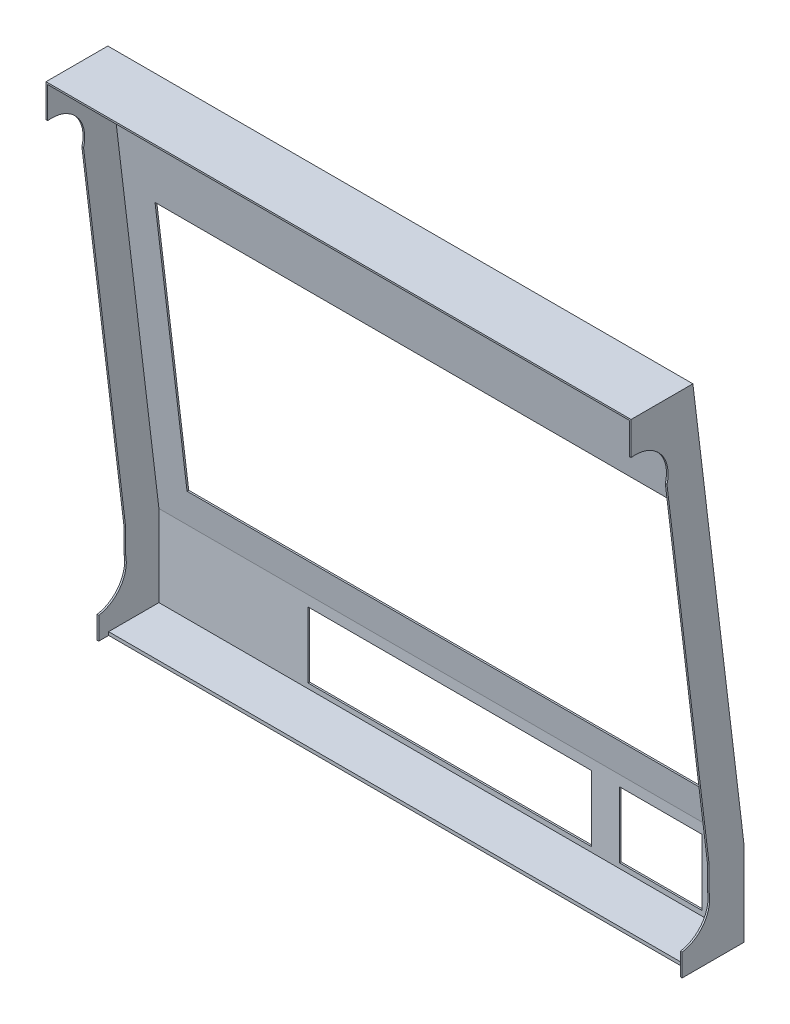
from build123d import *

# Parameters (mm, degrees)
BOSS_EXTRUDE1_DEPTH = 2
BOSS_EXTRUDE2_DEPTH = 706
SKETCH3_W           = 706
SKETCH3_H           = 73
CUT_EXTRUDE1_DEPTH  = 940.955850027
BOSS_EXTRUDE3_START = 2
BOSS_EXTRUDE3_DEPTH = 2
CUT_EXTRUDE2_REACH  = 951.714
SKETCH5_W           = 628
SKETCH5_H           = 323
SKETCH6_W           = 100
SKETCH6_H           = 80
SKETCH6_W_2         = 344
CUT_EXTRUDE3_DEPTH  = 2
SKETCH7_W           = 706
SKETCH7_H           = 4
BOSS_EXTRUDE4_DEPTH = 61


with BuildPart() as part:
    # Sketch1 → Boss-Extrude1 (new body)
    with BuildSketch(Plane(origin=(0, 0, 0), x_dir=(0, 0, -1), z_dir=(1, 0, 0))):
        with BuildLine():
            Line((0, 0), (-75, 0))
            Line((-75, 0), (-75, -40))
            ThreePointArc((-75, -40), (-39.844354311, -53.471133381), (-31.447716035, -90.171096924))
            Line((-31.447716035, -90.171096924), (19.696734432, -515))
            Line((19.696734432, -515), (19.696734432, -543.691772505))
            ThreePointArc((19.696734432, -543.691772505), (13.304376378, -574.16353688), (-13, -590.820981133))
            Line((-13, -590.820981133), (-13, -618))
            Line((-13, -618), (62, -618))
            Line((62, -618), (62, -515))
            Line((62, -515), (0, 0))
        make_face()
    extrude(amount=BOSS_EXTRUDE1_DEPTH)

    # Sketch2 → Boss-Extrude2 (add)
    with BuildSketch(Plane.ZY):
        Polygon((13, -618), (-62, -618), (-62, -515), (0, 0), (75, 0), (75, -2), (1.773664518, -2), (-60, -515.119955274), (-60, -616), (13, -616), align=None)
    extrude(amount=BOSS_EXTRUDE2_DEPTH)

    # Sketch3 → Cut-Extrude1 (cut, through all)
    with BuildSketch(Plane(origin=(0, -616, 0), x_dir=(1, 0, 0), z_dir=(0, 1, 0))):
        with Locations((-353, 23.5)):
            Rectangle(SKETCH3_W, SKETCH3_H)
    extrude(amount=-CUT_EXTRUDE1_DEPTH, mode=Mode.SUBTRACT)

    # Sketch4 → Boss-Extrude3 (add)
    with BuildSketch(Plane.ZY.offset(706).offset(BOSS_EXTRUDE3_START)):
        with BuildLine():
            Line((-19.696734432, -543.691772505), (-19.696734432, -515))
            Line((-19.696734432, -515), (31.447716035, -90.171096924))
            ThreePointArc((31.447716035, -90.171096924), (39.844354311, -53.471133381), (75, -40))
            Line((75, -40), (75, 0))
            Line((75, 0), (0, 0))
            Line((0, 0), (-62, -515))
            Line((-62, -515), (-62, -618))
            Line((-62, -618), (13, -618))
            Line((13, -618), (13, -590.820981133))
            ThreePointArc((13, -590.820981133), (-13.304376378, -574.16353688), (-19.696734432, -543.691772505))
        make_face()
    extrude(amount=-BOSS_EXTRUDE3_DEPTH)

    # Cut-Extrude2: up to this plane
    cut_extrude2_end = Plane(origin=(-706, -515.119955274, -60), z_dir=(0, 0.1195253040577556, -0.9928311546732914))
    # Sketch5 → Cut-Extrude2 (cut, up to the surface)
    with BuildSketch(Plane(origin=(0, 0, -62), x_dir=(-1, 0, 0), z_dir=(0, 0, -1)), mode=Mode.PRIVATE) as cut_extrude2_sk1:
        with Locations((353, -313.5)):
            Rectangle(SKETCH5_W, SKETCH5_H)
    cut_extrude2_tool1 = split(extrude(cut_extrude2_sk1.sketch, amount=-CUT_EXTRUDE2_REACH, mode=Mode.PRIVATE), bisect_by=cut_extrude2_end, keep=Keep.BOTH, mode=Mode.PRIVATE)
    add(cut_extrude2_tool1.solids().sort_by_distance((-353, -313.5, -62))[0], mode=Mode.SUBTRACT)

    # Sketch6 → Cut-Extrude3 (cut)
    with BuildSketch(Plane(origin=(0, 0, -62), x_dir=(-1, 0, 0), z_dir=(0, 0, -1))):
        with Locations((97, -568)):
            Rectangle(SKETCH6_W, SKETCH6_H)
        with Locations((353, -568)):
            Rectangle(SKETCH6_W_2, SKETCH6_H)
    extrude(amount=-CUT_EXTRUDE3_DEPTH, mode=Mode.SUBTRACT)

    # Sketch7 → Boss-Extrude4 (add)
    with BuildSketch(Plane.XY.offset(-60)):
        with Locations((-353, -616)):
            Rectangle(SKETCH7_W, SKETCH7_H)
    extrude(amount=BOSS_EXTRUDE4_DEPTH)


solid = part.part
